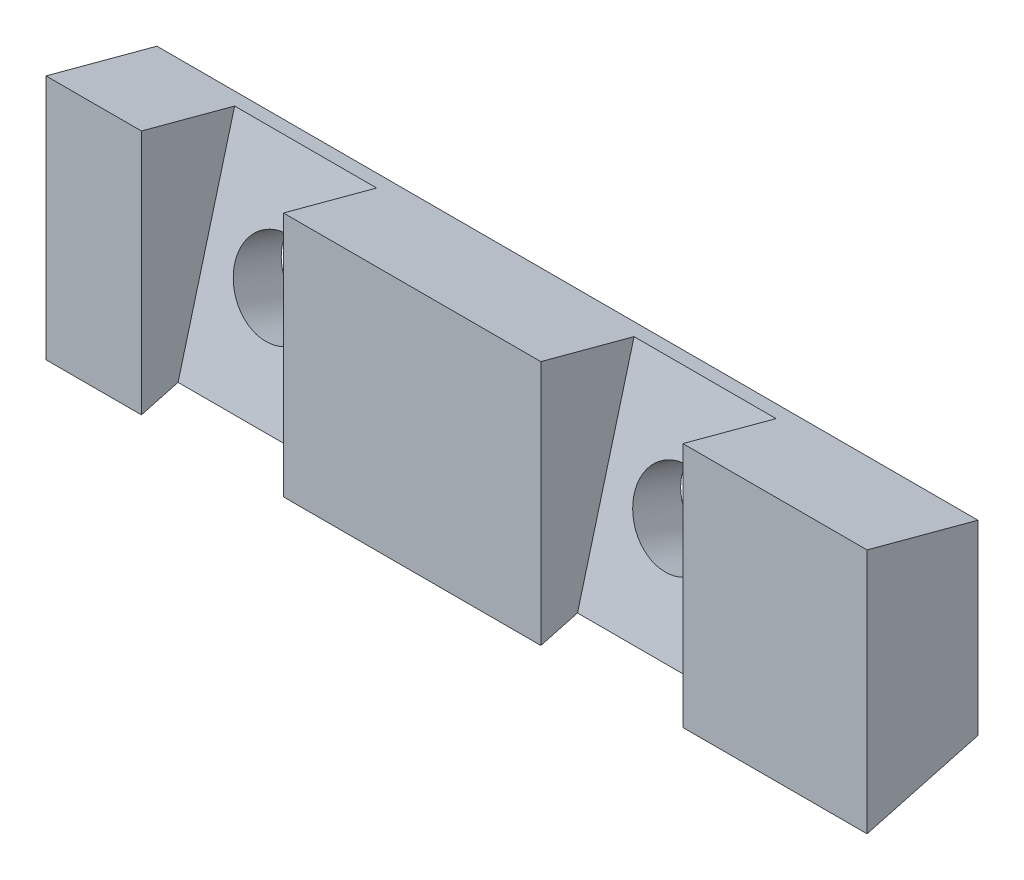
SolidWorks part; units mm, degrees
material "ZG120Mn13-2"
ref_plane "Front Plane" through (0, 0, 0) normal (0, 0, 1) x (1, 0, 0)
ref_plane "Top Plane" through (0, 0, 0) normal (0, 1, 0) x (1, 0, 0)
ref_plane "Right Plane" through (0, 0, 0) normal (1, 0, 0) x (0, 0, -1)
sketch "Sketch1" plane through (0, 0, 0) normal (1, 0, 0) x (0, 0, -1)
  line L0 (0, 0) -> (0, 110.7949)
  line L1 (0, 110.7949) -> (50, 97.3975)
  line L2 (50, 97.3975) -> (50, 13.3975)
  line L3 (50, 13.3975) -> (0, 0)
  line L4 (0, 55.3975) -> (-40.1546, 55.3975) construction
  dimension "D1" = 15
  dimension "D2" = 84
  dimension "D3" = 50
extrude "Boss-Extrude1" add sketch "Sketch1" along normal mid plane 370
sketch "Sketch2" plane through (-185, 0, 0) normal (-1, 0, 0) x (0, 0, 1)
  line L0 (0, 0) -> (-50, 0)
  line L1 (-50, 0) -> (-50, 13.3975)
  line L2 (-50, 13.3975) -> (0, 0)
extrude "Boss-Extrude2" add sketch "Sketch2" against normal blind 35
sketch "Sketch3" plane through (0, 0, 0) normal (1, 0, 0) x (0, 0, -1)
  line L0 (16.5173, 4.4258) -> (42.0032, 99.5402)
  line L1 (0, 0) -> (50, 13.3975) construction
  line L2 (50, 97.3975) -> (0, 110.7949) construction
  line L3 (42.0032, 99.5402) -> (0, 110.7949)
  line L4 (0, 110.7949) -> (0, 0)
  line L5 (0, 0) -> (16.5173, 4.4258)
  dimension "D1" = 15
  dimension "D2" = 17.1
extrude "Cut-Extrude1" cut sketch "Sketch3" against normal mid plane 64 from offset 110 offset against normal yes
sketch "Sketch4" plane through (0, 0, 0) normal (1, 0, 0) x (0, 0, -1)
  line L4 (16.5173, 4.4258) -> (42.0032, 99.5402)
  line L5 (42.0032, 99.5402) -> (0, 110.7949)
  line L6 (0, 110.7949) -> (0, 0)
  line L7 (0, 0) -> (16.5173, 4.4258)
  line L8 (16.5173, 4.4258) -> (42.0032, 99.5402)
  line L9 (42.0032, 99.5402) -> (0, 110.7949)
  line L10 (0, 110.7949) -> (0, 0)
  line L11 (0, 0) -> (16.5173, 4.4258)
  dimension "D1" = 0
extrude "Cut-Extrude2" cut sketch "Sketch4" against normal mid plane 64 from offset 70
sketch "Sketch5" plane through (0, 0, 0) normal (1, 0, 0) x (0, 0, -1)
  line L0 (-8.0454, 43.3975) -> (50, 43.3975) construction
  line L1 (50, 13.3975) -> (50, 97.3975) construction
  line L2 (50, 43.3975) -> (-23.6482, 70.2032)
  dimension "D1" = 30
  dimension "D2" = 20
ref_plane "Plane1" through (0, 54.3906, -19.7966) normal (0, 0.9397, -0.342) x (0, 0.342, 0.9397)
sketch "Sketch6" plane through (0, 54.3906, -19.7966) normal (0, 0.9397, -0.342) x (0, 0.342, 0.9397)
  line L0 (-67.9052, -110) -> (52.6032, -110) construction
  line L1 (-63.6028, -91) -> (12.8983, -91)
  line L2 (12.8983, -91) -> (12.8983, -110)
  line L3 (12.8983, -110) -> (-63.6028, -110)
  line L4 (-63.6028, -110) -> (-63.6028, -91)
  dimension "D1" = 40
  dimension "D2" = 19
revolve "Cut-Revolve1" cut sketch "Sketch6" angle 360 about L0
pattern_linear "LPattern1" count 2 spacing 180 along (1, 0, 0) of "Cut-Revolve1"
